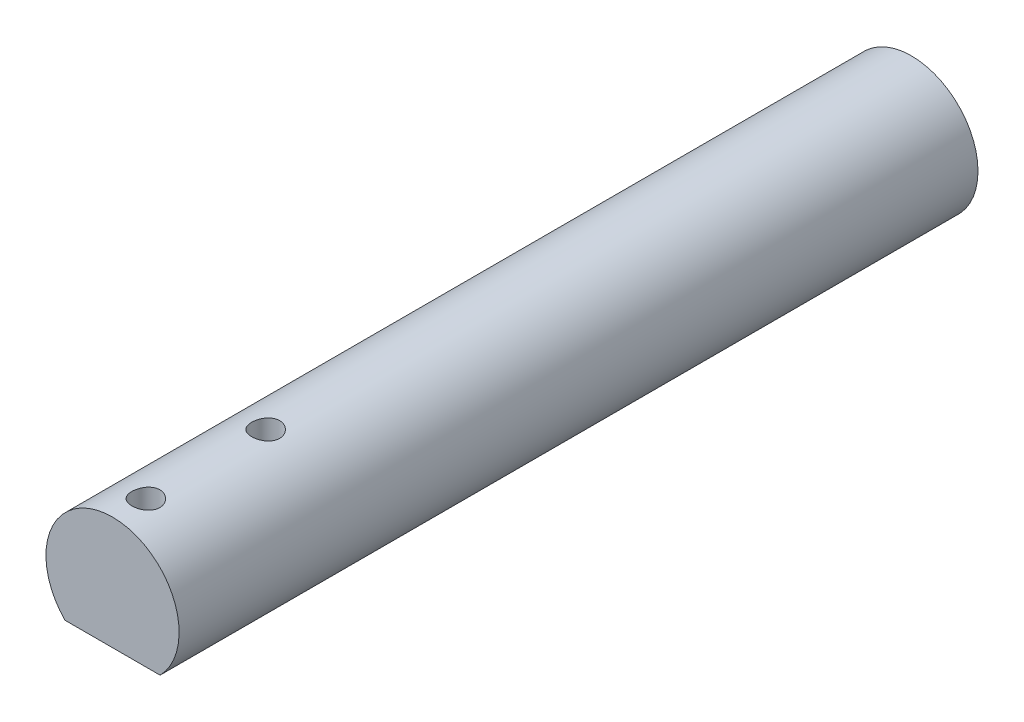
SolidWorks part; units mm, degrees
ref_plane "前视基准面" through (0, 0, 0) normal (0, 0, 1) x (1, 0, 0)
ref_plane "上视基准面" through (0, 0, 0) normal (0, 1, 0) x (1, 0, 0)
ref_plane "右视基准面" through (0, 0, 0) normal (1, 0, 0) x (0, 0, -1)
sketch "草图1" plane through (0, 0, 0) normal (0, 0, 1) x (1, 0, 0)
  circle A0 centre (0, 0) radius 10
  dimension "D1" = 20
extrude "凸台-拉伸1" add sketch "草图1" along normal mid plane 120
hole_wizard "M6 螺纹孔1" positions "草图2" profile "草图4" tap size "M6" standard "GB"
sketch "草图2" plane through (0, 0, -60) normal (0, 0, -1) x (-1, 0, 0)
  point P0 (0, 0)
sketch "草图4" plane through (0, 0, -60) normal (1, 0, 0) x (0, 1, 0)
  line L0 (0, 0) -> (0, 16.5022)
  line L1 (0, 16.5022) -> (2.5, 15)
  line L2 (2.5, 15) -> (2.5, 0)
  line L5 (2.5, 0) -> (0, 0)
  line L10 (0, 16.5022) -> (-2.5, 15) construction
  line L11 (0, -6.35) -> (0, 107.95) construction
  dimension "螺纹孔钻头直径" = 5
  dimension "螺纹孔钻头深度" = 15
  dimension "导头角度" = 118
sketch "草图5" plane through (0, 0, 60) normal (0, 0, 1) x (1, 0, 0)
  line L0 (0, 0) -> (0, -7) construction
  line L1 (7.1414, -13) -> (-7.1414, -13)
  line L2 (7.1414, -13) -> (7.1414, -7)
  line L3 (7.1414, -7) -> (-7.1414, -7)
  line L4 (-7.1414, -13) -> (-7.1414, -7)
  line L5 (7.1414, -13) -> (-7.1414, -7) construction
  line L6 (7.1414, -7) -> (-7.1414, -13) construction
  circle A0 centre (0, 0) radius 10 construction
  point P0 (0, -10)
  dimension "D1" = 6
extrude "切除-拉伸1" cut sketch "草图5" against normal blind 30
hole_wizard "M5 螺纹孔1" positions "草图6" profile "草图7" tap size "M5" standard "GB" end condition up to next
sketch "草图6" plane through (0, -7, 0) normal (0, -1, 0) x (-1, 0, 0)
  line L0 (0, -60) -> (0, -55) construction
  line L1 (-7.1414, -60) -> (7.1414, -60) construction
  line L2 (0, -55) -> (0, -37) construction
  point P0 (0, -55)
  point P2 (0, -37)
  dimension "D1" = 18
  dimension "D2" = 5
sketch "草图7" plane through (0, -7, 55) normal (1, 0, 0) x (0, 0, -1)
  line L0 (0, 0) -> (0, 17)
  line L1 (0, 17) -> (2.1, 17)
  line L2 (2.1, 17) -> (2.1, 0)
  line L5 (2.1, 0) -> (0, 0)
  line L11 (0, -6.35) -> (0, 107.95) construction
  dimension "通孔螺纹孔钻头直径" = 4.2
  dimension "通孔螺纹孔钻头深度" = 17
